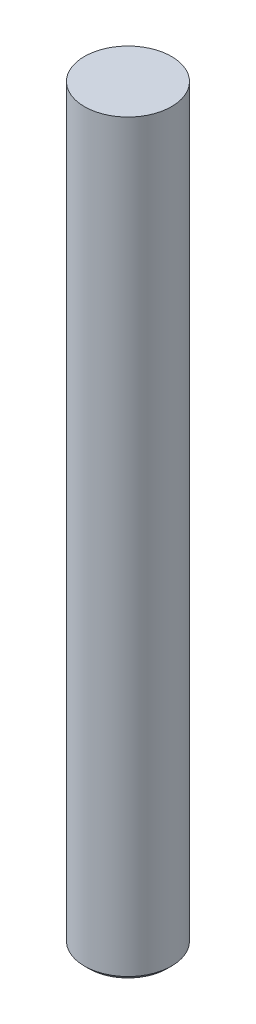
SolidWorks part; units mm, degrees
ref_plane "Front Plane" through (0, 0, 0) normal (0, 0, 1) x (1, 0, 0)
ref_plane "Top Plane" through (0, 0, 0) normal (0, 1, 0) x (1, 0, 0)
ref_plane "Right Plane" through (0, 0, 0) normal (1, 0, 0) x (0, 0, -1)
sketch "Sketch2" plane through (0, 0, 0) normal (0, 1, 0) x (1, 0, 0)
  circle A0 centre (0, 0) radius 10
  dimension "D1" = 20
extrude "Boss-Extrude1" add sketch "Sketch2" along normal blind 172
cosmetic thread "Cosmetic Thread1" parameters "D1"=40, "D2"=17.294
chamfer "Chamfer1" distance 1 angle 45 1 edges at (0, 0, 10)
